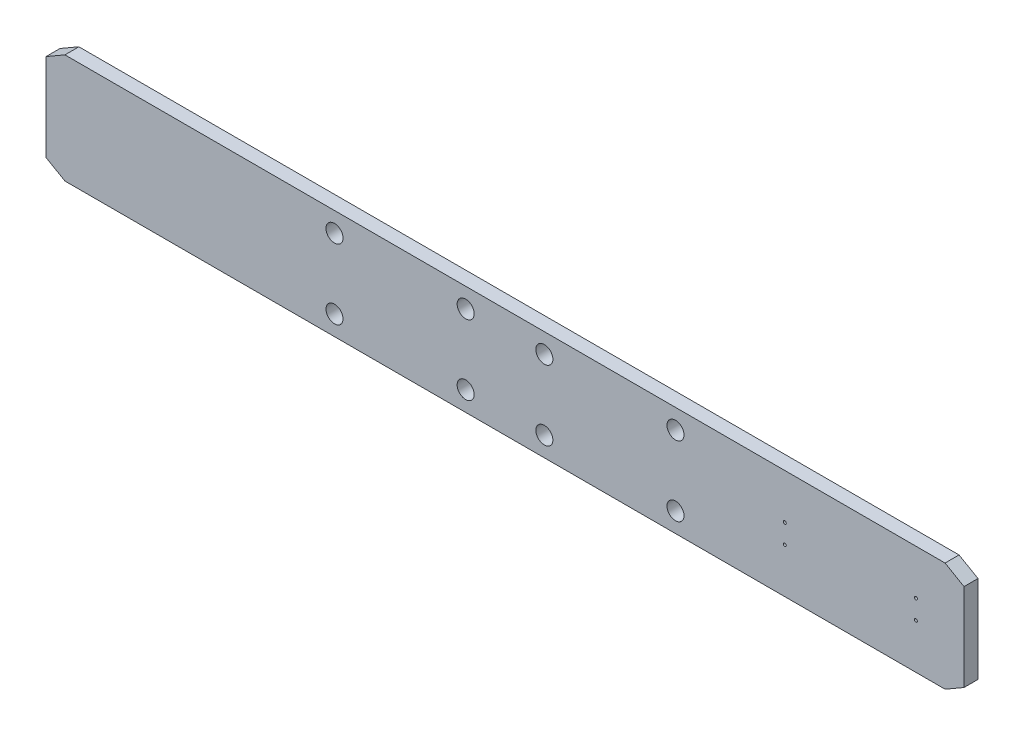
from build123d import *

# Parameters (mm, degrees)
SKETCH1_R            = 19.5
BOSS_EXTRUDE1_DEPTH  = 16
M8_TAPPED_HOLE1_D    = 6.8
LPATTERN1_COUNT      = 2
LPATTERN1_PITCH      = 300
LPATTERN1_COUNT_DIR2 = 2
LPATTERN1_PITCH_DIR2 = 44


with BuildPart() as part:
    # Sketch1 → Boss-Extrude1 (new, symmetric)
    with BuildSketch(Plane.XY):
        Polygon((1050, 100), (1006.698729811, 125), (-1006.698729811, 125), (-1050, 100), (-1050, -100), (-1006.698729811, -125), (1006.698729811, -125), (1050, -100), align=None)
        with Locations((-390, 80)):
            Circle(SKETCH1_R, mode=Mode.SUBTRACT)
        with Locations((-90, 80)):
            Circle(SKETCH1_R, mode=Mode.SUBTRACT)
        with Locations(Location((-90, -80, 0), (0, 0, 180))):
            Circle(SKETCH1_R, mode=Mode.SUBTRACT)
        with Locations(Location((-390, -80, 0), (0, 0, 180))):
            Circle(SKETCH1_R, mode=Mode.SUBTRACT)
        with Locations((390, -80)):
            Circle(SKETCH1_R, mode=Mode.SUBTRACT)
        with Locations((90, -80)):
            Circle(SKETCH1_R, mode=Mode.SUBTRACT)
        with Locations(Location((90, 80, 0), (0, 0, 180))):
            Circle(SKETCH1_R, mode=Mode.SUBTRACT)
        with Locations(Location((390, 80, 0), (0, 0, 180))):
            Circle(SKETCH1_R, mode=Mode.SUBTRACT)
    extrude(amount=BOSS_EXTRUDE1_DEPTH, both=True)

    # M8 Tapped Hole1 (through all)
    with Locations(Plane.XY.offset(16)):
        with Locations((640, 22)):
            m8_tapped_hole1 = Hole(M8_TAPPED_HOLE1_D / 2)

    # LPattern1: M8 Tapped Hole1 2 × 2
    with Locations(*[(i * LPATTERN1_PITCH, -j * LPATTERN1_PITCH_DIR2, 0) for i in range(LPATTERN1_COUNT) for j in range(LPATTERN1_COUNT_DIR2) if (i, j) != (0, 0)]):
        add(m8_tapped_hole1, mode=Mode.SUBTRACT)


solid = part.part
